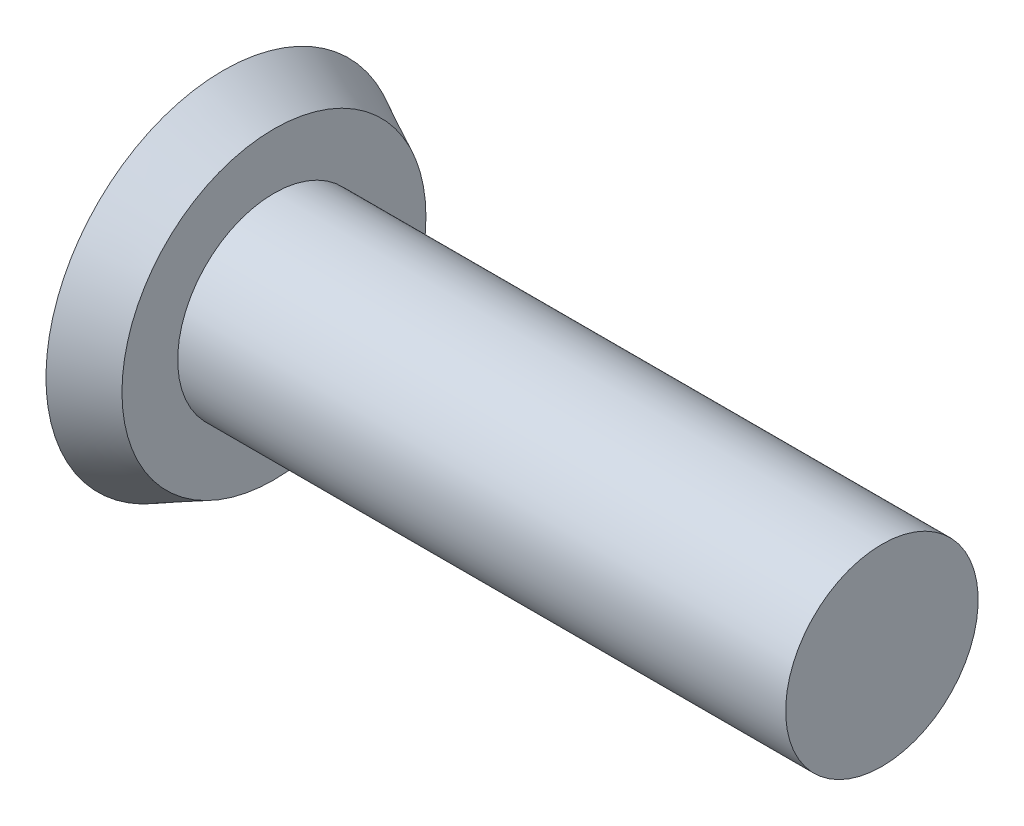
SolidWorks part; units mm, degrees
ref_plane "Front Plane" through (0, 0, 0) normal (0, 0, 1) x (1, 0, 0)
ref_plane "Top Plane" through (0, 0, 0) normal (0, 1, 0) x (1, 0, 0)
ref_plane "Right Plane" through (0, 0, 0) normal (1, 0, 0) x (0, 0, -1)
other "Configuration Table"
sketch "Sketch1" plane through (0, 0, 0) normal (0, 0, 1) x (1, 0, 0)
  line L0 (0, 0) -> (0, 3.5)
  line L1 (0, 3.5) -> (1, 3)
  line L2 (1, 3) -> (1, 1.9)
  line L3 (1, 1.9) -> (13, 1.9)
  line L4 (13, 1.9) -> (13, 0)
  line L5 (13, 0) -> (0, 0) construction
  line L6 (0, 0) -> (13, 0)
  dimension "D1" = 13
  dimension "D2" = 1
  dimension "D3" = 3.8
  dimension "D4" = 7
  dimension "D5" = 6
revolve "Revolve1" add sketch "Sketch1" angle 360 about L5
